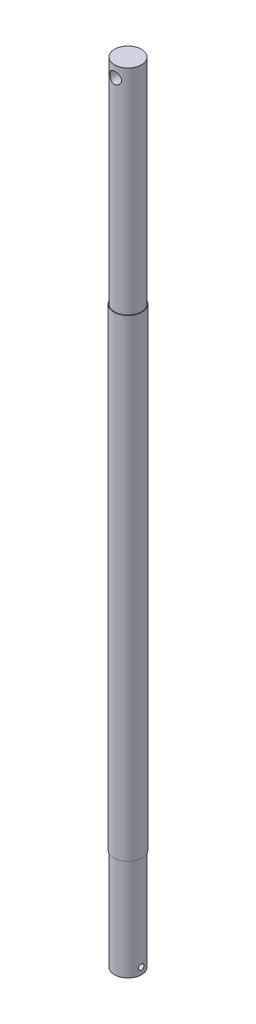
from build123d import *

# Parameters (mm, degrees)
SKETCH1_R               = 12
BOSS_EXTRUDE1_DEPTH     = 90
SKETCH2_R               = 12.5
BOSS_EXTRUDE2_DEPTH     = 420
SKETCH3_R               = 12
BOSS_EXTRUDE3_DEPTH     = 190
CUT_EXTRUDE1_DEPTH      = 701.223178708
CUT_EXTRUDE1_DEPTH_BACK = 701.223178708
SKETCH4_R               = 5.1
CUT_EXTRUDE2_DEPTH      = 701.223178808
CUT_EXTRUDE2_DEPTH_BACK = 701.223178808
SKETCH5_R               = 2.5


with BuildPart() as part:
    # Sketch1 → Boss-Extrude1 (new body)
    with BuildSketch(Plane(origin=(0, 0, 0), x_dir=(1, 0, 0), z_dir=(0, 1, 0))):
        with Locations(Location((0, 0, 0), (0, 0, 90))):
            Circle(SKETCH1_R)
    extrude(amount=BOSS_EXTRUDE1_DEPTH)

    # Sketch2 → Boss-Extrude2 (add)
    with BuildSketch(Plane(origin=(0, 90, 0), x_dir=(1, 0, 0), z_dir=(0, 1, 0))):
        with Locations(Location((0, 0, 0), (0, 0, 270))):
            Circle(SKETCH2_R)
    extrude(amount=BOSS_EXTRUDE2_DEPTH)

    # Sketch3 → Boss-Extrude3 (add)
    with BuildSketch(Plane(origin=(0, 510, 0), x_dir=(1, 0, 0), z_dir=(0, 1, 0))):
        with Locations(Location((0, 0, 0), (0, 0, 90))):
            Circle(SKETCH3_R)
    extrude(amount=BOSS_EXTRUDE3_DEPTH)

    # Sketch4 → Cut-Extrude1 (cut, two sides: drawn at the far end of the back side and taken through both)
    with BuildSketch(Plane.XY.offset(-CUT_EXTRUDE1_DEPTH_BACK)):
        with Locations(Location((0, 690, 0), (0, 0, 90))):
            Circle(SKETCH4_R)
    extrude(amount=CUT_EXTRUDE1_DEPTH + CUT_EXTRUDE1_DEPTH_BACK, mode=Mode.SUBTRACT)

    # Sketch5 → Cut-Extrude2 (cut, two sides: drawn at the far end of the back side and taken through both)
    with BuildSketch(Plane(origin=(0, 0, 0), x_dir=(0, 0, -1), z_dir=(1, 0, 0)).offset(-CUT_EXTRUDE2_DEPTH_BACK)):
        with Locations((0, 6)):
            Circle(SKETCH5_R)
    extrude(amount=CUT_EXTRUDE2_DEPTH + CUT_EXTRUDE2_DEPTH_BACK, mode=Mode.SUBTRACT)


solid = part.part
